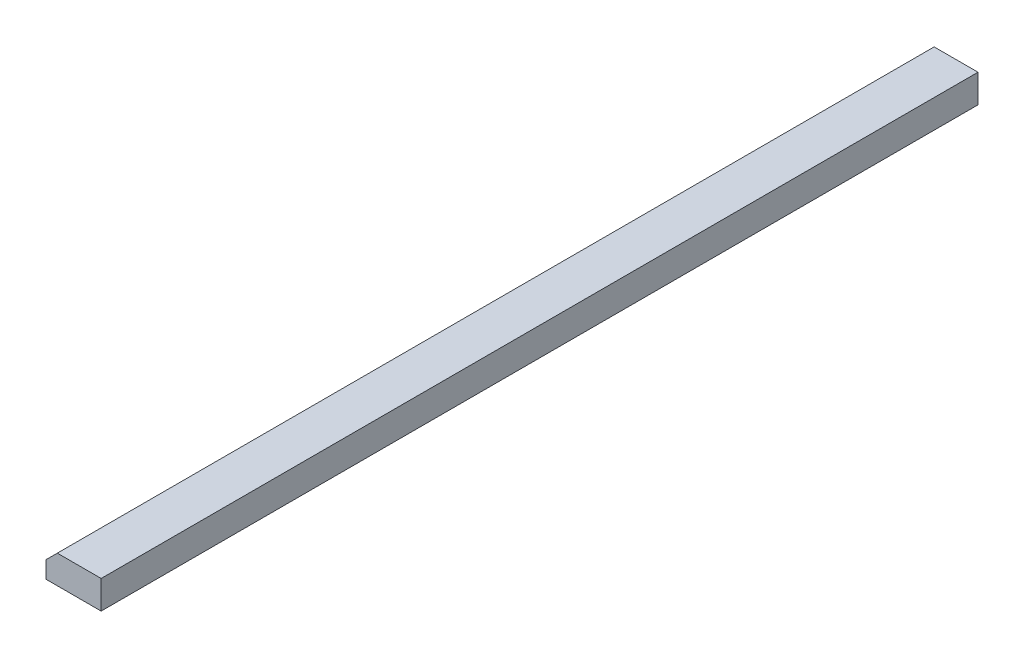
SolidWorks part; units mm, degrees
ref_plane "Front Plane" through (0, 0, 0) normal (0, 0, 1) x (1, 0, 0)
ref_plane "Top Plane" through (0, 0, 0) normal (0, 1, 0) x (1, 0, 0)
ref_plane "Right Plane" through (0, 0, 0) normal (1, 0, 0) x (0, 0, -1)
sketch "Sketch1" plane through (0, 0, 0) normal (0, 0, 1) x (1, 0, 0)
  line L1 (0, 0) -> (39, 0)
  line L2 (0, 0) -> (0, 20)
  line L3 (0, 20) -> (39, 20)
  line L4 (39, 0) -> (39, 20)
  dimension "D1" = 20
  dimension "D2" = 39
extrude "Boss-Extrude1" add sketch "Sketch1" along normal blind 620
chamfer "Chamfer1" distance 8 angle 45 1 edges at (0, 20, 310)
